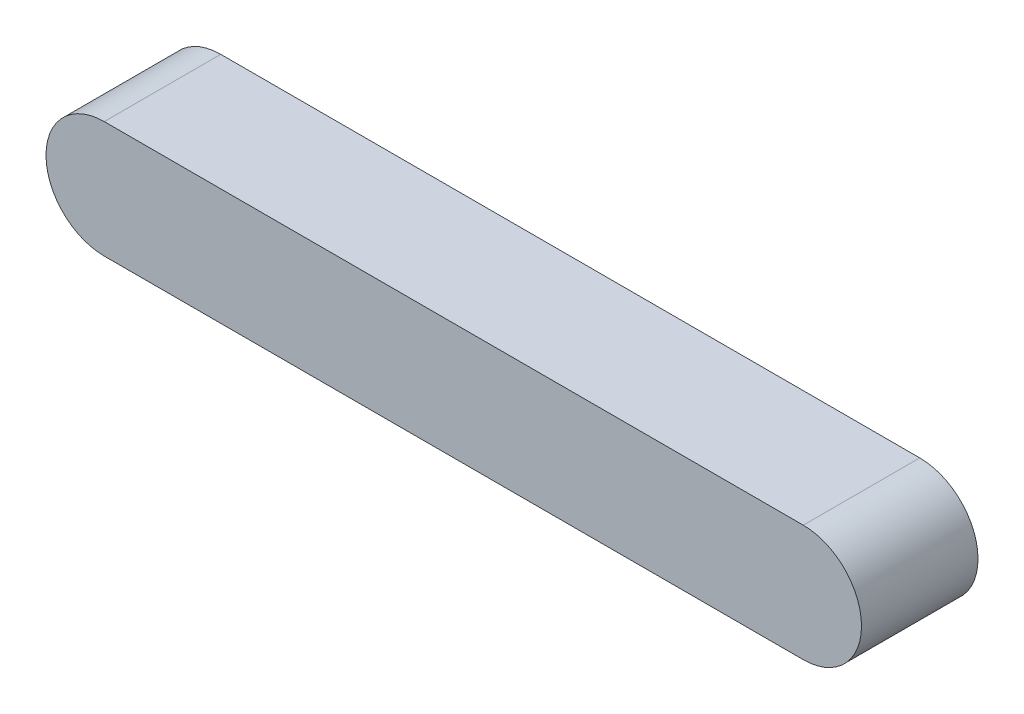
SolidWorks part; units mm, degrees
ref_plane "Front Plane" through (0, 0, 0) normal (0, 0, 1) x (1, 0, 0)
ref_plane "Top Plane" through (0, 0, 0) normal (0, 1, 0) x (1, 0, 0)
ref_plane "Right Plane" through (0, 0, 0) normal (1, 0, 0) x (0, 0, -1)
other "Configuration Table"
sketch "Sketch1" plane through (0, 0, 0) normal (0, 0, 1) x (1, 0, 0)
  line L0 (-15, 0) -> (15, 0) construction
  line L1 (-15, 2.5) -> (15, 2.5)
  line L2 (-15, -2.5) -> (15, -2.5)
  arc A0 (-15, 2.5) -> (-15, -2.5) centre (-15, 0) ccw
  arc A1 (15, -2.5) -> (15, 2.5) centre (15, 0) ccw
  point P2 (0, 0)
  dimension "D1" = 5
  dimension "D2" = 30
extrude "Boss-Extrude1" add sketch "Sketch1" along normal blind 5
